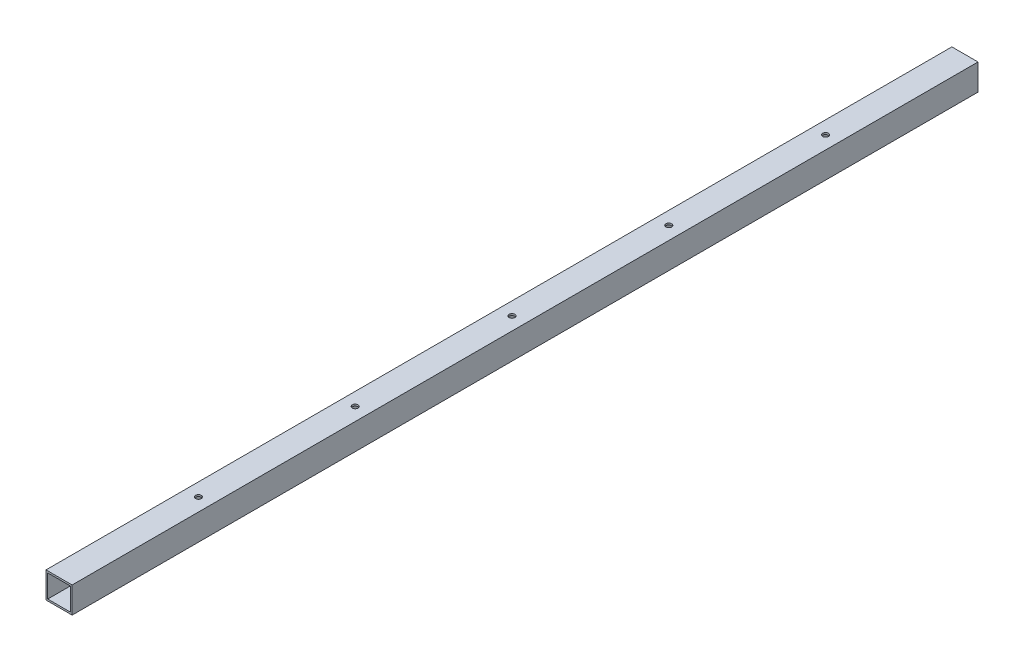
from build123d import *

# Parameters (mm, degrees)
SKETCH_1_W          = 30
SKETCH_1_H          = 30
SKETCH_1_W_2        = 26
SKETCH_1_H_2        = 26
EXTRUDE_1_DEPTH     = 520
SKETCH_3_R          = 3.3
CUT_EXTRUDE_1_DEPTH = 636


with BuildPart() as part:
    # 草图1 → 凸台-拉伸1 (new, symmetric)
    with BuildSketch(Plane.XY):
        Rectangle(SKETCH_1_W, SKETCH_1_H)
        Rectangle(SKETCH_1_W_2, SKETCH_1_H_2, mode=Mode.SUBTRACT)
    extrude(amount=EXTRUDE_1_DEPTH, both=True)

    # 草图3 → 切除-拉伸1 (cut)
    with BuildSketch(Plane(origin=(0, 15, 0), x_dir=(1, 0, 0), z_dir=(0, 1, 0))):
        with Locations(Location((0, 360, 0), (0, 0, 270))):
            Circle(SKETCH_3_R)
        with Locations(Location((0, 180, 0), (0, 0, 270))):
            Circle(SKETCH_3_R)
        with Locations(Location((0, 0, 0), (0, 0, 270))):
            Circle(SKETCH_3_R)
        with Locations(Location((0, -180, 0), (0, 0, 270))):
            Circle(SKETCH_3_R)
        with Locations(Location((0, -360, 0), (0, 0, 270))):
            Circle(SKETCH_3_R)
    extrude(amount=-CUT_EXTRUDE_1_DEPTH, mode=Mode.SUBTRACT)


solid = part.part
